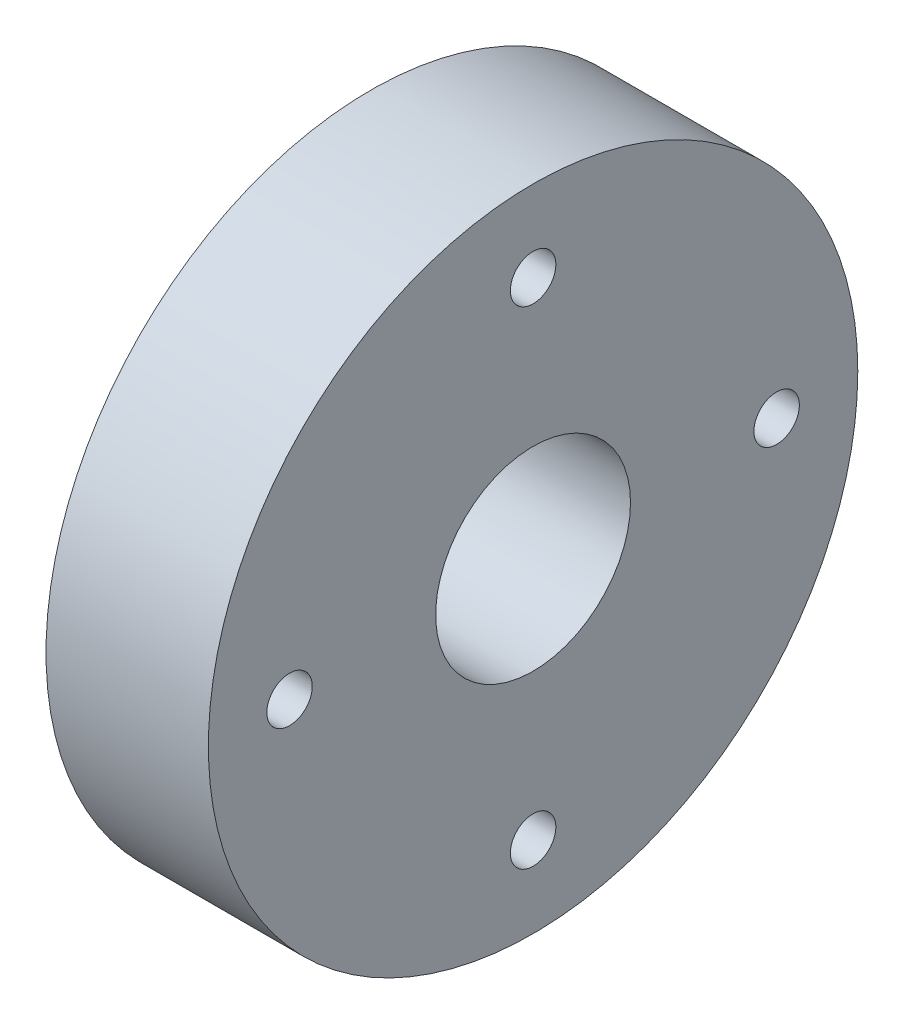
SolidWorks part; units mm, degrees
material "AISI 1045 钢，冷拔"
ref_plane "Front Plane" through (0, 0, 0) normal (0, 0, 1) x (1, 0, 0)
ref_plane "Top Plane" through (0, 0, 0) normal (0, 1, 0) x (1, 0, 0)
ref_plane "Right Plane" through (0, 0, 0) normal (1, 0, 0) x (0, 0, -1)
sketch "Sketch1" plane through (0, 0, 0) normal (0, 0, 1) x (1, 0, 0)
  line L0 (71.9012, 0) -> (0, 0) construction
  line L1 (0, 0) -> (0, 101.4822) construction
  line L3 (-25, 30) -> (25, 30)
  line L4 (-25, 30) -> (-25, 100)
  line L5 (-25, 100) -> (25, 100)
  line L6 (25, 30) -> (25, 100)
  line L7 (-25, 30) -> (25, 100) construction
  line L8 (-25, 100) -> (25, 30) construction
  point P3 (0, 65)
  dimension "D1" = 50
  dimension "D2" = 200
  dimension "D3" = 60
revolve "Revolve1" add sketch "Sketch1" angle 360 about L0
sketch "Sketch3" plane through (-25, 0, 0) normal (-1, 0, 0) x (0, 0, 1)
  line L0 (0, 0) -> (-75, 0) construction
  circle A0 centre (0, 0) radius 75
  dimension "D1" = 150
hole_wizard "M16 Tapped Hole1" positions "3DSketch2" profile "Sketch4" tap size "M16" standard "GB" end condition through all
sketch3d "3DSketch2"
  point P0 (-25, 0, -75)
sketch "Sketch4" plane through (-25, 0, -75) normal (0, 1, 0) x (0, 0, 1)
  line L0 (0, 0) -> (0, 50)
  line L1 (0, 50) -> (7, 50)
  line L2 (7, 50) -> (7, 0)
  line L5 (7, 0) -> (0, 0)
  line L11 (0, -6.35) -> (0, 107.95) construction
  dimension "通孔螺纹孔钻头直径" = 14
  dimension "通孔螺纹孔钻头深度" = 50
cosmetic thread "Cosmetic thread1" parameters "D2"=16
pattern_circular "CirPattern1" count 4 over 360 about axis through (0, 0, 0) along (1, 0, 0) of "M16 Tapped Hole1"
